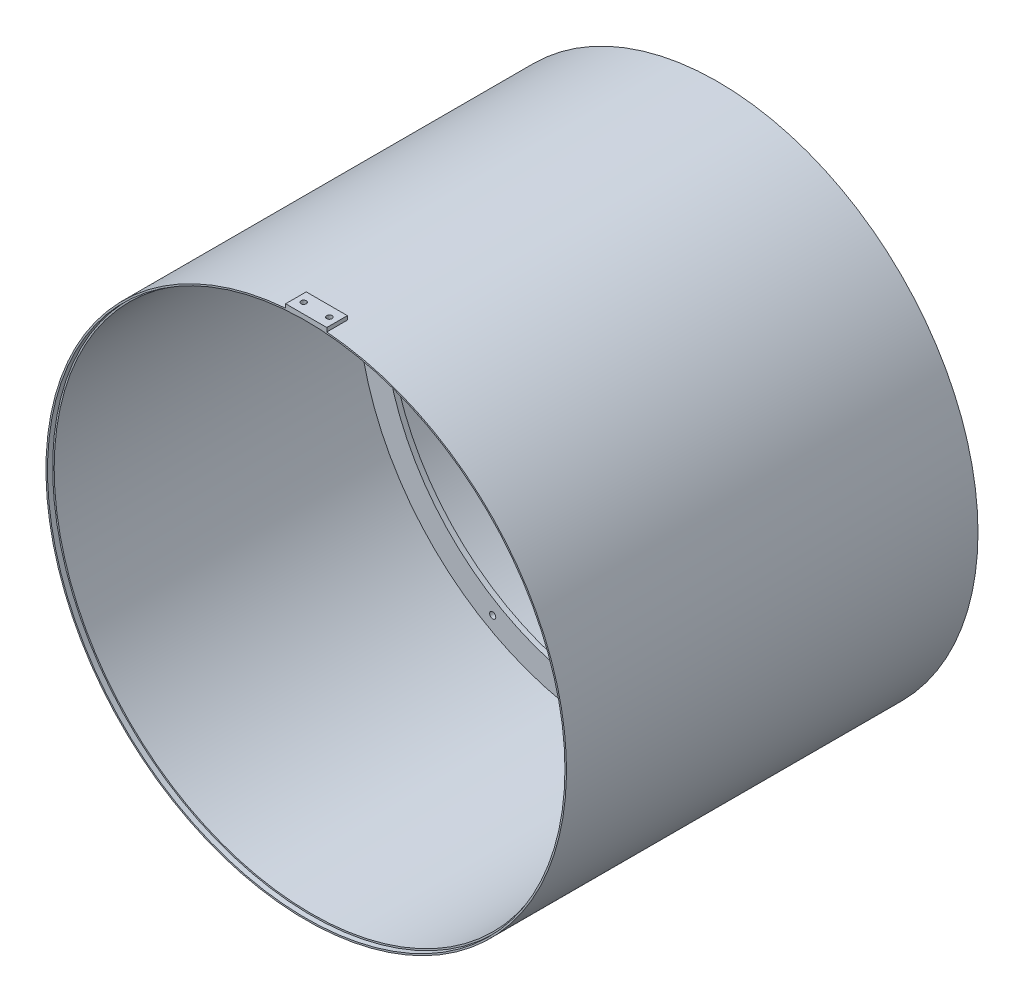
from build123d import *

# Parameters (mm, degrees)
SKETCH1_R                = 253
SKETCH1_R_2              = 250
BOSS_EXTRUDE1_DEPTH      = 400
BOSS_EXTRUDE2_START      = -95
SKETCH2_R                = 250
SKETCH2_R_2              = 225
BOSS_EXTRUDE2_DEPTH      = 5
SKETCH3_R                = 3
CUT_EXTRUDE1_DEPTH       = 20
CIRPATTERN1_COUNT        = 6
BOSS_EXTRUDE4_REACH      = 697.047
BOSS_EXTRUDE4_END_RADIUS = 253
SKETCH6_W                = 40
SKETCH6_H                = 20
CUT_EXTRUDE2_REACH       = 697.047
CUT_EXTRUDE2_END_RADIUS  = 250
SKETCH8_R                = 2.604926317
CUT_EXTRUDE3_START       = -5
SKETCH9_R                = 251.5
SKETCH9_R_2              = 250
CUT_EXTRUDE3_DEPTH       = 5


with BuildPart() as part:
    # Sketch1 → Boss-Extrude1 (new body)
    with BuildSketch(Plane.XY):
        Circle(SKETCH1_R)
        Circle(SKETCH1_R_2, mode=Mode.SUBTRACT)
    extrude(amount=BOSS_EXTRUDE1_DEPTH)

    # Sketch2 → Boss-Extrude2 (add)
    with BuildSketch(Plane(origin=(0, 0, 0), x_dir=(-1, 0, 0), z_dir=(0, 0, -1)).offset(BOSS_EXTRUDE2_START)):
        Circle(SKETCH2_R)
        Circle(SKETCH2_R_2, mode=Mode.SUBTRACT)
    extrude(amount=-BOSS_EXTRUDE2_DEPTH)

    # Sketch3 → Cut-Extrude1 (cut)
    with BuildSketch(Plane(origin=(0, 0, 95), x_dir=(-1, 0, 0), z_dir=(0, 0, -1))):
        with Locations((237.5, 0)):
            Circle(SKETCH3_R)
    cut_extrude1 = extrude(amount=-CUT_EXTRUDE1_DEPTH, mode=Mode.SUBTRACT)

    # CirPattern1: Cut-Extrude1 ×6 about axis
    cirpattern1_axis = Axis((0, 0, 0), (0, 0, 1))
    for i in range(1, CIRPATTERN1_COUNT):
        add(cut_extrude1.rotate(cirpattern1_axis, i * 360 / CIRPATTERN1_COUNT), mode=Mode.SUBTRACT)

    # Boss-Extrude4: up to this cylinder (the profile starts outside it)
    boss_extrude4_end = Plane(origin=(0, 0, 390), z_dir=(0, 0, -1)) * Cylinder(BOSS_EXTRUDE4_END_RADIUS, 1901.094, mode=Mode.PRIVATE)
    # Sketch6 → Boss-Extrude4 (add, up to the surface)
    with BuildSketch(Plane(origin=(0, 256, 0), x_dir=(1, 0, 0), z_dir=(0, 1, 0)), mode=Mode.PRIVATE) as boss_extrude4_sk1:
        with Locations((0, -390)):
            Rectangle(SKETCH6_W, SKETCH6_H)
    boss_extrude4_tool1 = extrude(boss_extrude4_sk1.sketch, amount=-BOSS_EXTRUDE4_REACH, mode=Mode.PRIVATE) - boss_extrude4_end
    add(boss_extrude4_tool1.solids().sort_by_distance((0, 256, 390))[0])

    # Cut-Extrude2: up to this cylinder (the profile starts outside it)
    cut_extrude2_end = Plane(origin=(0, 0, 390), z_dir=(0, 0, -1)) * Cylinder(CUT_EXTRUDE2_END_RADIUS, 1895.094, mode=Mode.PRIVATE)
    # Sketch8 → Cut-Extrude2 (cut, up to the surface)
    with BuildSketch(Plane(origin=(0, 256, 0), x_dir=(1, 0, 0), z_dir=(0, 1, 0)), mode=Mode.PRIVATE) as cut_extrude2_sk1:
        with Locations(Location((-12.5, -390, 0), (0, 0, 270))):
            Circle(SKETCH8_R)
    cut_extrude2_tool1 = extrude(cut_extrude2_sk1.sketch, amount=-CUT_EXTRUDE2_REACH, mode=Mode.PRIVATE) - cut_extrude2_end
    add(cut_extrude2_tool1.solids().sort_by_distance((-12.5, 256, 390))[0], mode=Mode.SUBTRACT)
    # Sketch8 → Cut-Extrude2 (cut, up to the surface)
    with BuildSketch(Plane(origin=(0, 256, 0), x_dir=(1, 0, 0), z_dir=(0, 1, 0)), mode=Mode.PRIVATE) as cut_extrude2_sk2:
        with Locations(Location((12.5, -390, 0), (0, 0, 270))):
            Circle(SKETCH8_R)
    cut_extrude2_tool2 = extrude(cut_extrude2_sk2.sketch, amount=-CUT_EXTRUDE2_REACH, mode=Mode.PRIVATE) - cut_extrude2_end
    add(cut_extrude2_tool2.solids().sort_by_distance((12.5, 256, 390))[0], mode=Mode.SUBTRACT)

    # Sketch9 → Cut-Extrude3 (cut)
    with BuildSketch(Plane.XY.offset(400).offset(CUT_EXTRUDE3_START)):
        Circle(SKETCH9_R)
        with Locations(Location((0, 0, 0), (0, 0, 180))):
            Circle(SKETCH9_R_2, mode=Mode.SUBTRACT)
    extrude(amount=CUT_EXTRUDE3_DEPTH, mode=Mode.SUBTRACT)


solid = part.part
